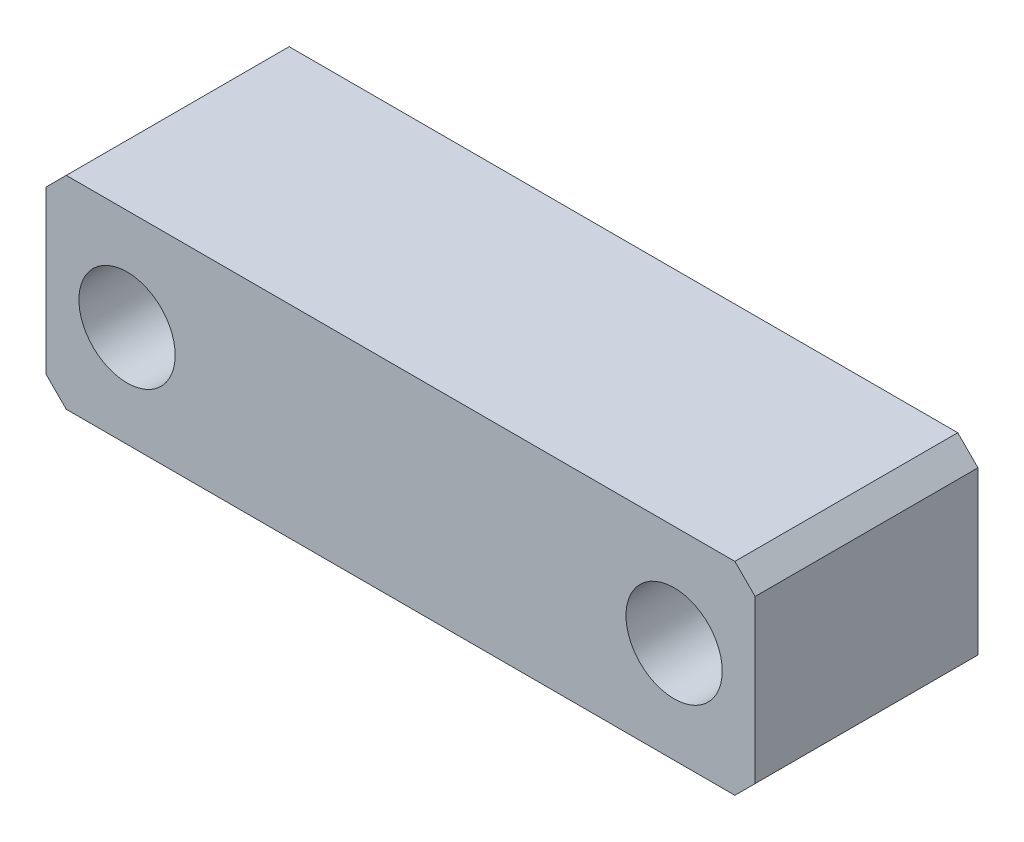
from build123d import *

# Parameters (mm, degrees)
BOSS_EXTRUDE1_DEPTH      = 10
BOSS_EXTRUDE1_DEPTH_BACK = 12
SKETCH1_W                = 70
SKETCH1_H                = 20
SKETCH1_R                = 2.187999439
SKETCH1_R_2              = 2.181063018
HOLE1_D                  = 6
HOLE1_CBORE_D            = 9.5
HOLE1_CBORE_DEPTH        = 8.5
CHAMFER1_SIZE            = 2


with BuildPart() as part:
    # Sketch1 → Boss-Extrude1 (new, two sides: drawn at the far end of the back side and taken through both)
    with BuildSketch(Plane.XY.offset(-BOSS_EXTRUDE1_DEPTH_BACK)):
        with Locations((2.309691162, 2.003205128)):
            Rectangle(SKETCH1_W, SKETCH1_H)
        with Locations((-24.690308838, 2.003205128)):
            Circle(SKETCH1_R, mode=Mode.SUBTRACT)
        with Locations((29.309691162, 2.003205128)):
            Circle(SKETCH1_R_2, mode=Mode.SUBTRACT)
    extrude(amount=BOSS_EXTRUDE1_DEPTH + BOSS_EXTRUDE1_DEPTH_BACK)

    # Hole1 (through all)
    with Locations(Plane.XY.offset(10)):
        with Locations((-24.690308838, 2.003205128), (29.309691162, 2.003205128)):
            CounterBoreHole(HOLE1_D / 2, HOLE1_CBORE_D / 2, HOLE1_CBORE_DEPTH)

    # Chamfer1
    chamfer1_edges = [part.edges().sort_by_distance(p)[0] for p in [
        (-32.690308838, 12.003205128, -1),
        (37.309691162, 12.003205128, -1),
        (37.309691162, -7.996794872, -1),
        (-32.690308838, -7.996794872, -1),
    ]]
    chamfer(chamfer1_edges, length=CHAMFER1_SIZE)


solid = part.part
